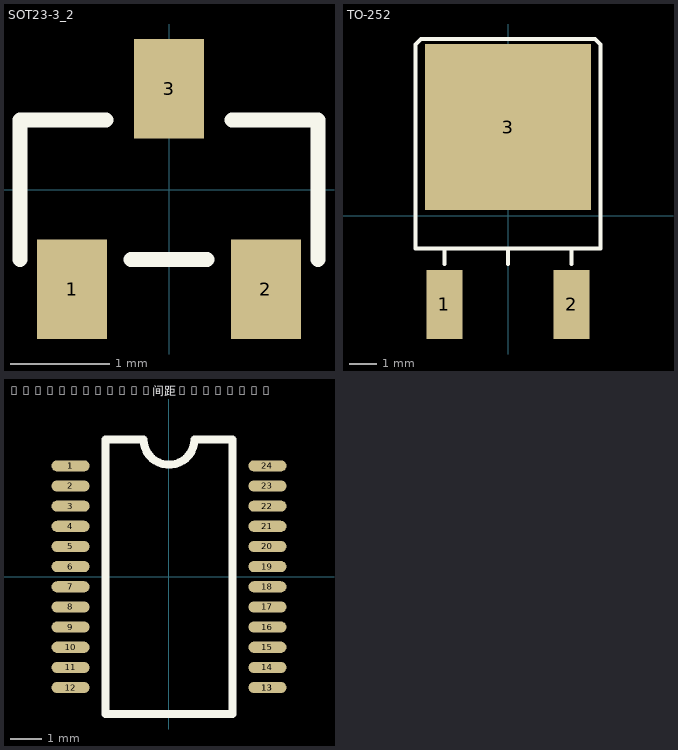
[diagram p0: the footprints below, top view; thin cyan lines are the x and y axes]
# Altium footprint library MISC84401-2.PcbLib: 19 footprints (part 2 of 2)
Each footprint in its own frame and in the unit in brackets; x right, y up, seen from the top. Pads: shape width x height; smd on the part's side, far side on the other; paste and mask are expansions set on the pad; w line width, h text height; cw(c..) or ccw(c..) is an arc to the next point about the centre after c.

## SOT23-3_2 [mm]
pads (3):
  rect 0.7x1 smd: 1(-0.975,-1) 2(0.975,-1) 3(0,1.016)
Top Overlay:
  lines w0.15: -1.5,-0.7 -1.5,0.7 -0.635,0.7 ; -0.381,-0.7 0.381,-0.7 ; 0.635,0.7 1.5,0.7 1.5,-0.7

## TO-252 [mm]
height 1.75
pads (3):
  rect 1.3x2.5 smd: 1(-2.3,-3.212) 2(2.3,-3.212)
  rect 6x6 smd: 3(0,3.213)
Top Overlay:
  lines w0.15: -2.3,-1.75 -2.3,-1.18 ; 0,-1.75 0,-1.18 ; 2.3,-1.75 2.3,-1.18 ; -3.35,-1.18 -3.35,6.2 -3.15,6.4 3.15,6.4 3.35,6.2 3.35,6.19 3.35,-1.18 -3.35,-1.18

## TSSOP-24(pin间距0.635mm) [mm] "SMD IC"
height 10
pads (26):
  oval 1.2x0.35 smd: 1(-3.1,3.492) 1(-3.1,3.492) 2(-3.1,2.857) 3(-3.1,2.222) 4(-3.1,1.587) 5(-3.1,0.953) 6(-3.1,0.318) 7(-3.1,-0.318) 8(-3.1,-0.953) 9(-3.1,-1.587) 10(-3.1,-2.222) 11(-3.1,-2.857) 12(-3.1,-3.492) 13(3.1,-3.492) 13(3.1,-3.492) 14(3.1,-2.857) 15(3.1,-2.222) 16(3.1,-1.587) 17(3.1,-0.953) 18(3.1,-0.318) 19(3.1,0.318) 20(3.1,0.953) 21(3.1,1.587) 22(3.1,2.222) 23(3.1,2.857) 24(3.1,3.492)
Top Overlay:
  lines w0.254: -2,-4.325 2,-4.325 2,4.325 0.8,4.325 cw(c0,4.325) -0.8,4.325 -2,4.325 -2,-4.325